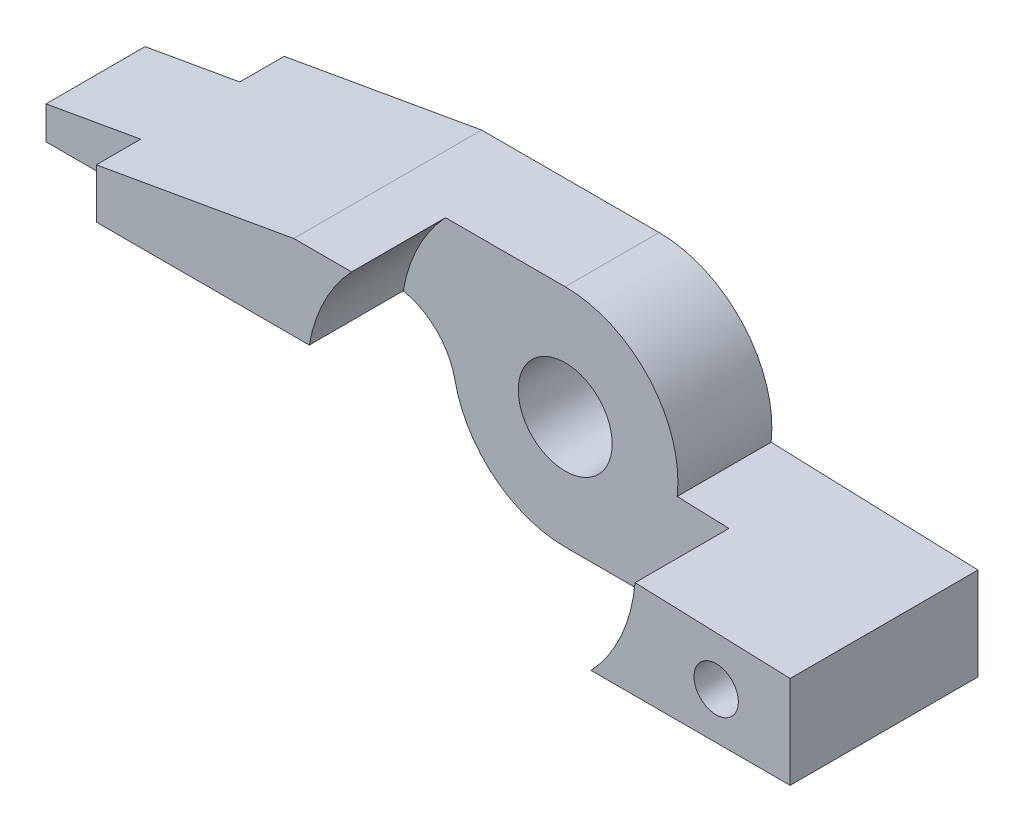
SolidWorks part; units mm, degrees
ref_plane "Front Plane" through (0, 0, 0) normal (0, 0, 1) x (1, 0, 0)
ref_plane "Top Plane" through (0, 0, 0) normal (0, 1, 0) x (1, 0, 0)
ref_plane "Right Plane" through (0, 0, 0) normal (1, 0, 0) x (0, 0, -1)
sketch "Sketch1" plane through (0, 0, 0) normal (0, 0, 1) x (1, 0, 0)
  line L0 (222.469, -15.24) -> (-101.1556, -15.24) construction
  line L1 (169.0764, 15.24) -> (-190.7542, 15.24) construction
  line L2 (165.1, -15.24) -> (165.1, -6.98)
  line L3 (165.1, -15.24) -> (0, -15.24)
  line L4 (165.1, -6.98) -> (22.141, -1.9878)
  line L5 (165.1, -6.98) -> (165.1, 34.4351) construction
  line L6 (0, 15.24) -> (-24, 15.24)
  line L7 (-24, 15.24) -> (-63.5, 8.26)
  line L8 (-63.5, 8.26) -> (-63.5, 0)
  line L9 (-63.5, 0) -> (-50.8, 0)
  line L10 (-46.99, 3.81) -> (-21.9011, 3.81)
  line L11 (10.0016, 0) -> (-11.8436, 0) construction
  line L12 (27.7905, -2.185) -> (15.14, -1.7433)
  line L13 (-50.8, 0) -> (-50.8, 3.81)
  line L14 (-50.8, 3.81) -> (-46.99, 3.81)
  circle A0 centre (0, 0) radius 6.35
  arc A1 (-14.921, -3.1019) -> (0, -15.24) centre (0, 0) ccw
  arc A2 (15.14, -1.7433) -> (0, 15.24) centre (0, 0) ccw
  arc A4 (-21.9011, 3.81) -> (-14.921, -3.1019) centre (-23.6249, -4.9113) cw
  dimension "D1" = 12.7
  dimension "D4" = 30.48
  dimension "D12" = 8.89
  dimension "D3" = 165.1
  dimension "D5" = 8.26
  dimension "D6" = 88
  dimension "D7" = 24
  dimension "D8" = 39.5
  dimension "D9" = 8.26
  dimension "D10" = 12.7
extrude "Boss-Extrude1" add sketch "Sketch1" along normal blind 25.4
sketch "Sketch2" plane through (0, 0, 25.4) normal (0, 0, 1) x (1, 0, 0)
  circle A0 centre (0, 0) radius 22.23
  dimension "D1" = 44.46
extrude "Cut-Extrude1" cut sketch "Sketch2" against normal blind 12.7
sketch "草图1" plane through (0, 0, 25.4) normal (0, 0, 1) x (1, 0, 0)
  line L0 (43.1091, -15.24) -> (43.1091, -2.72)
  line L1 (165.1, -6.98) -> (22.141, -1.9878) construction
  line L2 (43.1091, -2.72) -> (165.1, -6.98)
  line L3 (165.1, -6.98) -> (165.1, -15.24)
  line L4 (165.1, -15.24) -> (43.1091, -15.24)
  line L5 (165.1, -15.24) -> (16.1838, -15.24) construction
extrude "切除-拉伸1" cut sketch "草图1" against normal up to next
scale "缩放比例1" scale about origin uniform scaling yes scale factor 0.5
scale "缩放比例2" scale about origin uniform scaling yes scale factor 0.5
sketch "草图2" plane through (0, 0, 6.35) normal (0, 0, 1) x (1, 0, 0)
  line L0 (10.7773, -0.68) -> (10.7773, -3.81) construction
  line L1 (10.7773, -3.81) -> (4.0459, -3.81) construction
  circle A0 centre (8.2773, -2.245) radius 0.75
  point P4 (10.7773, -2.245)
  dimension "D1" = 1.5
  dimension "D2" = 2.5
  dimension "D3" = 1.565
extrude "切除-拉伸2" cut sketch "草图2" against normal through all
sketch "草图3" plane through (0, 0, 6.35) normal (0, 0, 1) x (1, 0, 0)
  line L0 (-15.875, 0.9525) -> (-15.875, 0)
  line L1 (-15.875, 0) -> (-12.7, 0)
  line L2 (-12.7, 0) -> (-12.7, 0.9525)
  line L5 (-12.7, 0.9525) -> (-15.875, 0.9525)
extrude "切除-拉伸3" cut sketch "草图3" against normal up to surface (6.35 mm away) up to face at (9.0273, -2.245, 0)
sketch "草图4" plane through (0, 0, 6.35) normal (0, 0, 1) x (1, 0, 0)
  line L0 (-15.875, 2.065) -> (-15.875, 0.9525)
  line L1 (-15.875, 0.9525) -> (-12.675, 0.9525)
  line L2 (-15.875, 0.9525) -> (-5.4753, 0.9525) construction
  line L3 (-12.675, 0.9525) -> (-12.675, 2.6305)
  line L4 (-6, 3.81) -> (-15.875, 2.065) construction
  line L5 (-12.675, 2.6305) -> (-15.875, 2.065)
  dimension "D1" = 3.2
extrude "切除-拉伸4" cut sketch "草图4" against normal blind 1.5
sketch "草图5" plane through (0, 0, 0) normal (0, 0, -1) x (-1, 0, 0)
  line L0 (15.875, 2.065) -> (15.875, 0.9525)
  line L1 (12.675, 0.9525) -> (15.875, 0.9525)
  line L3 (12.675, 2.6305) -> (12.675, 0.9525)
  line L4 (12.675, 2.6305) -> (15.875, 2.065)
extrude "切除-拉伸5" cut sketch "草图5" against normal blind 1.5
